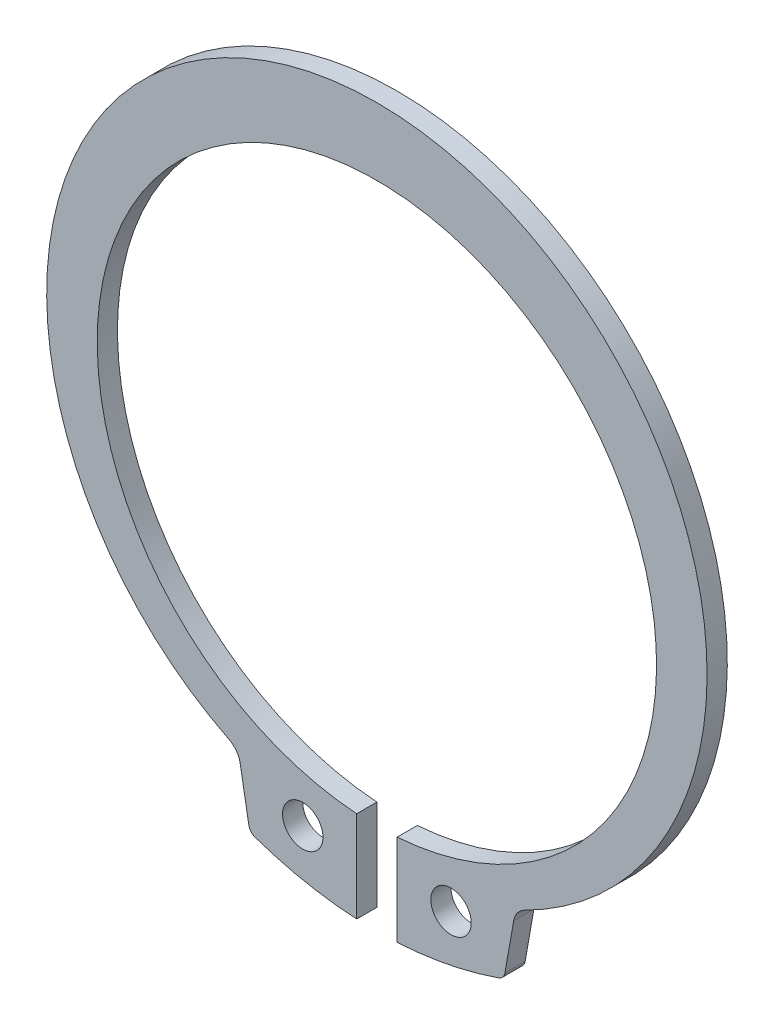
from build123d import *

# Parameters (mm, degrees)
EXTRUDE_972_DEPTH      = 0.75
EXTRUDE_972_DEPTH_BACK = 0.75
SKETCH_1_R             = 1.5


with BuildPart() as part:
    # 草图1 → Extrude 972 (new, two sides: drawn at the far end of the back side and taken through both)
    with BuildSketch(Plane.XY.offset(-EXTRUDE_972_DEPTH_BACK)):
        with BuildLine():
            Line((-1.5, -21.945712116), (-1.5, -28.709060435))
            ThreePointArc((-1.5, -28.709060435), (-5.322611287, -28.229989049), (-9.040763088, -27.22141896))
            ThreePointArc((-9.040763088, -27.22141896), (-9.343684575, -27.01404373), (-9.5, -26.68188202))
            Line((-9.5, -26.68188202), (-10.150143719, -22.994733766))
            ThreePointArc((-10.150143719, -22.994733766), (-10.42496916, -22.358396436), (-10.956546386, -21.91355953))
            ThreePointArc((-10.956546386, -21.91355953), (0, 24.5), (10.956546386, -21.91355953))
            ThreePointArc((10.956546386, -21.91355953), (10.42496916, -22.358396436), (10.150143719, -22.994733766))
            Line((10.150143719, -22.994733766), (9.5, -26.68188202))
            ThreePointArc((9.5, -26.68188202), (9.343684575, -27.01404373), (9.040763088, -27.22141896))
            ThreePointArc((9.040763088, -27.22141896), (5.322611287, -28.229989049), (1.5, -28.709060435))
            Line((1.5, -28.709060435), (1.5, -21.945712116))
            ThreePointArc((1.5, -21.945712116), (0, 19.5), (-1.5, -21.945712116))
        make_face()
        with Locations((-5.5, -24.714015002)):
            Circle(SKETCH_1_R, mode=Mode.SUBTRACT)
        with Locations(Location((5.5, -24.714015002, 0), (0, 0, 180))):
            Circle(SKETCH_1_R, mode=Mode.SUBTRACT)
    extrude(amount=EXTRUDE_972_DEPTH + EXTRUDE_972_DEPTH_BACK)


solid = part.part
